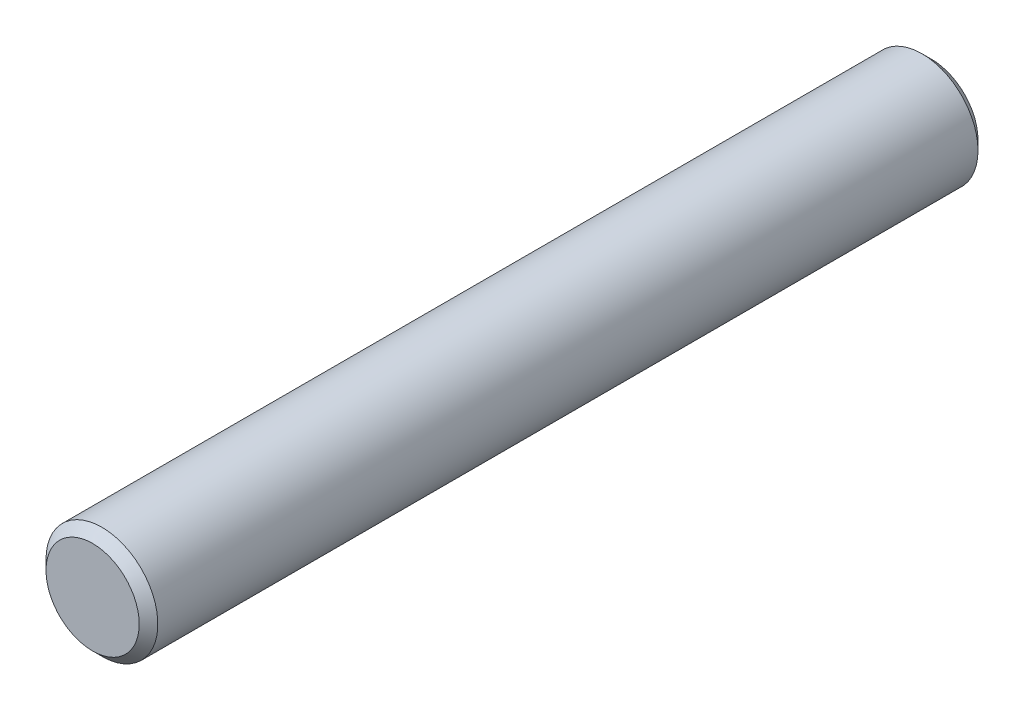
SolidWorks part; units mm, degrees
ref_plane "前视基准面" through (0, 0, 0) normal (0, 0, 1) x (1, 0, 0)
ref_plane "上视基准面" through (0, 0, 0) normal (0, 1, 0) x (1, 0, 0)
ref_plane "右视基准面" through (0, 0, 0) normal (1, 0, 0) x (0, 0, -1)
sketch "草图1" plane through (0, 0, 0) normal (0, 0, 1) x (1, 0, 0)
  circle A0 centre (0, 0) radius 3
  dimension "D1" = 6
extrude "凸台-拉伸1" add sketch "草图1" along normal blind 45
hole_wizard "M3 螺纹孔1" positions "草图3" profile "草图5" tap size "M3" standard "AS"
sketch "草图3" plane through (0, 0, 0) normal (0, 0, -1) x (-1, 0, 0)
  point P0 (0, 0)
sketch "草图5" plane through (0, 0, 0) normal (1, 0, 0) x (0, 1, 0)
  line L0 (0, 0) -> (0, 8.2511)
  line L1 (0, 8.2511) -> (1.25, 7.5)
  line L2 (1.25, 7.5) -> (1.25, 0)
  line L5 (1.25, 0) -> (0, 0)
  line L10 (0, 8.2511) -> (-1.25, 7.5) construction
  line L11 (0, -6.35) -> (0, 107.95) construction
  dimension "螺纹孔钻头直径" = 2.5
  dimension "螺纹孔钻头深度" = 7.5
  dimension "导头角度" = 118
cosmetic thread "孔螺蚊线1" parameters "D1"=6, "D2"=3
chamfer "倒角1" distance 0.5 angle 45 2 edges at (3, 0, 45) (3, 0, 0)
